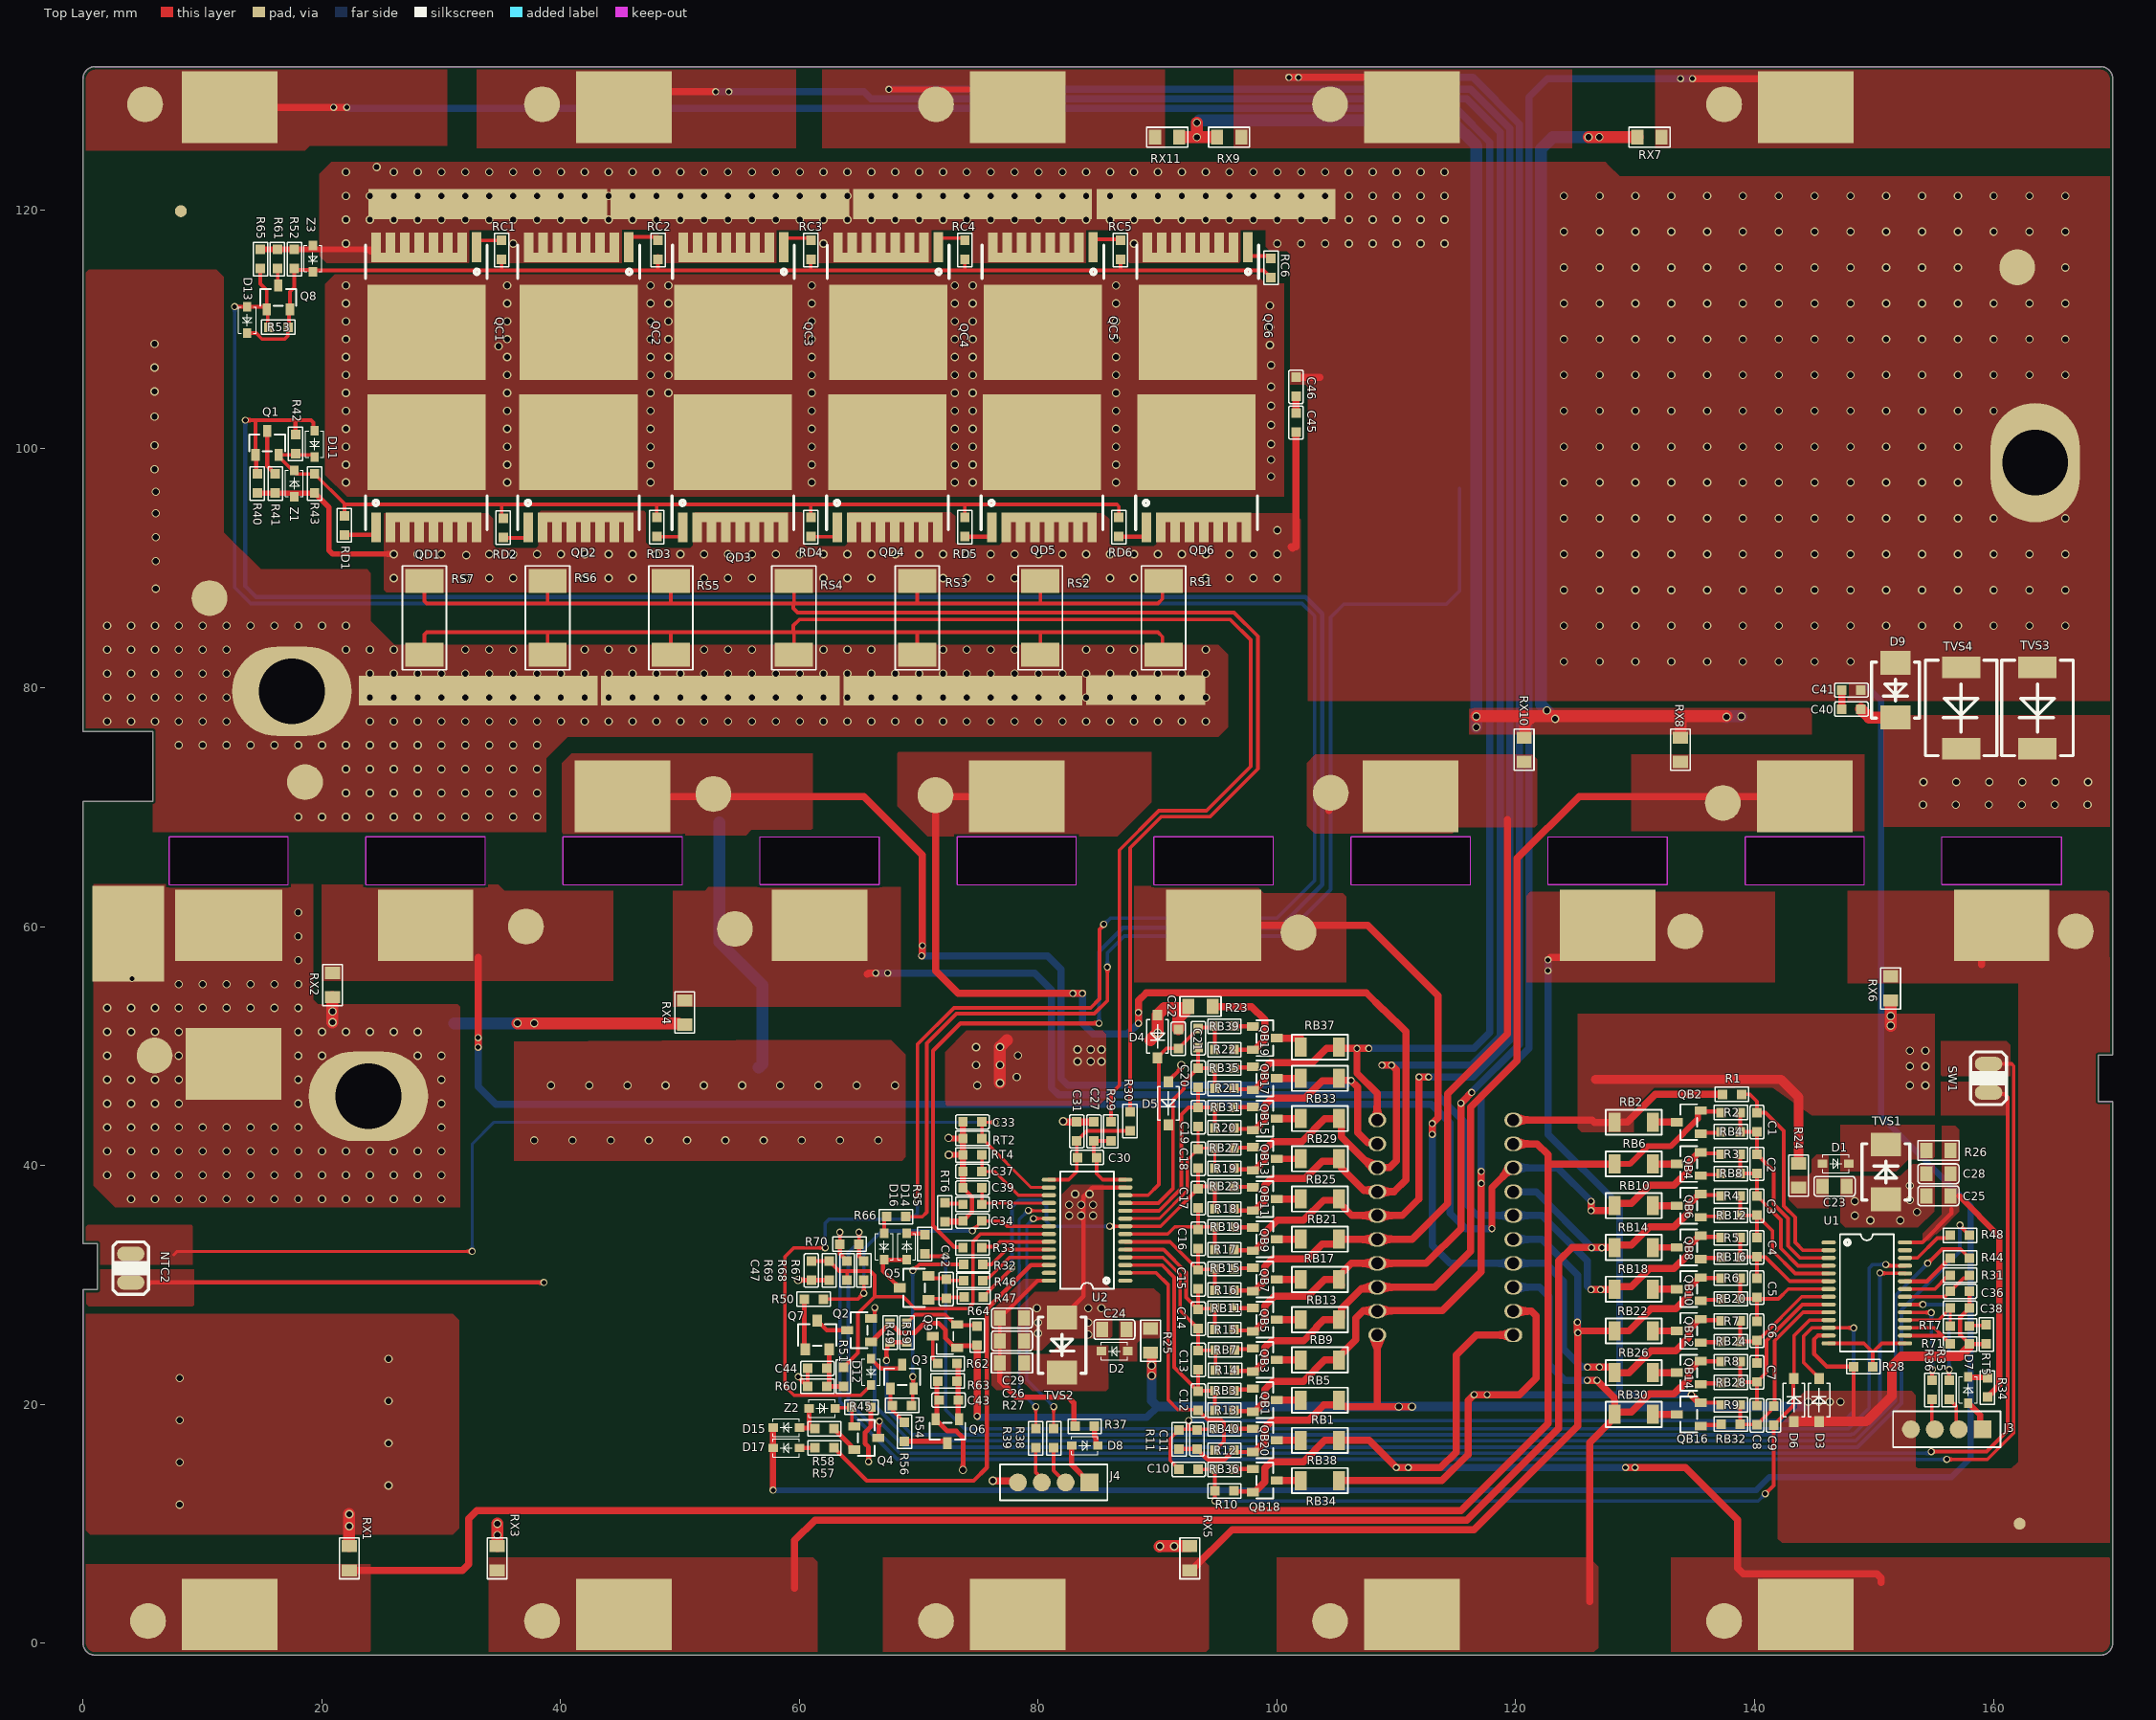
[diagram p0: Top Layer view]
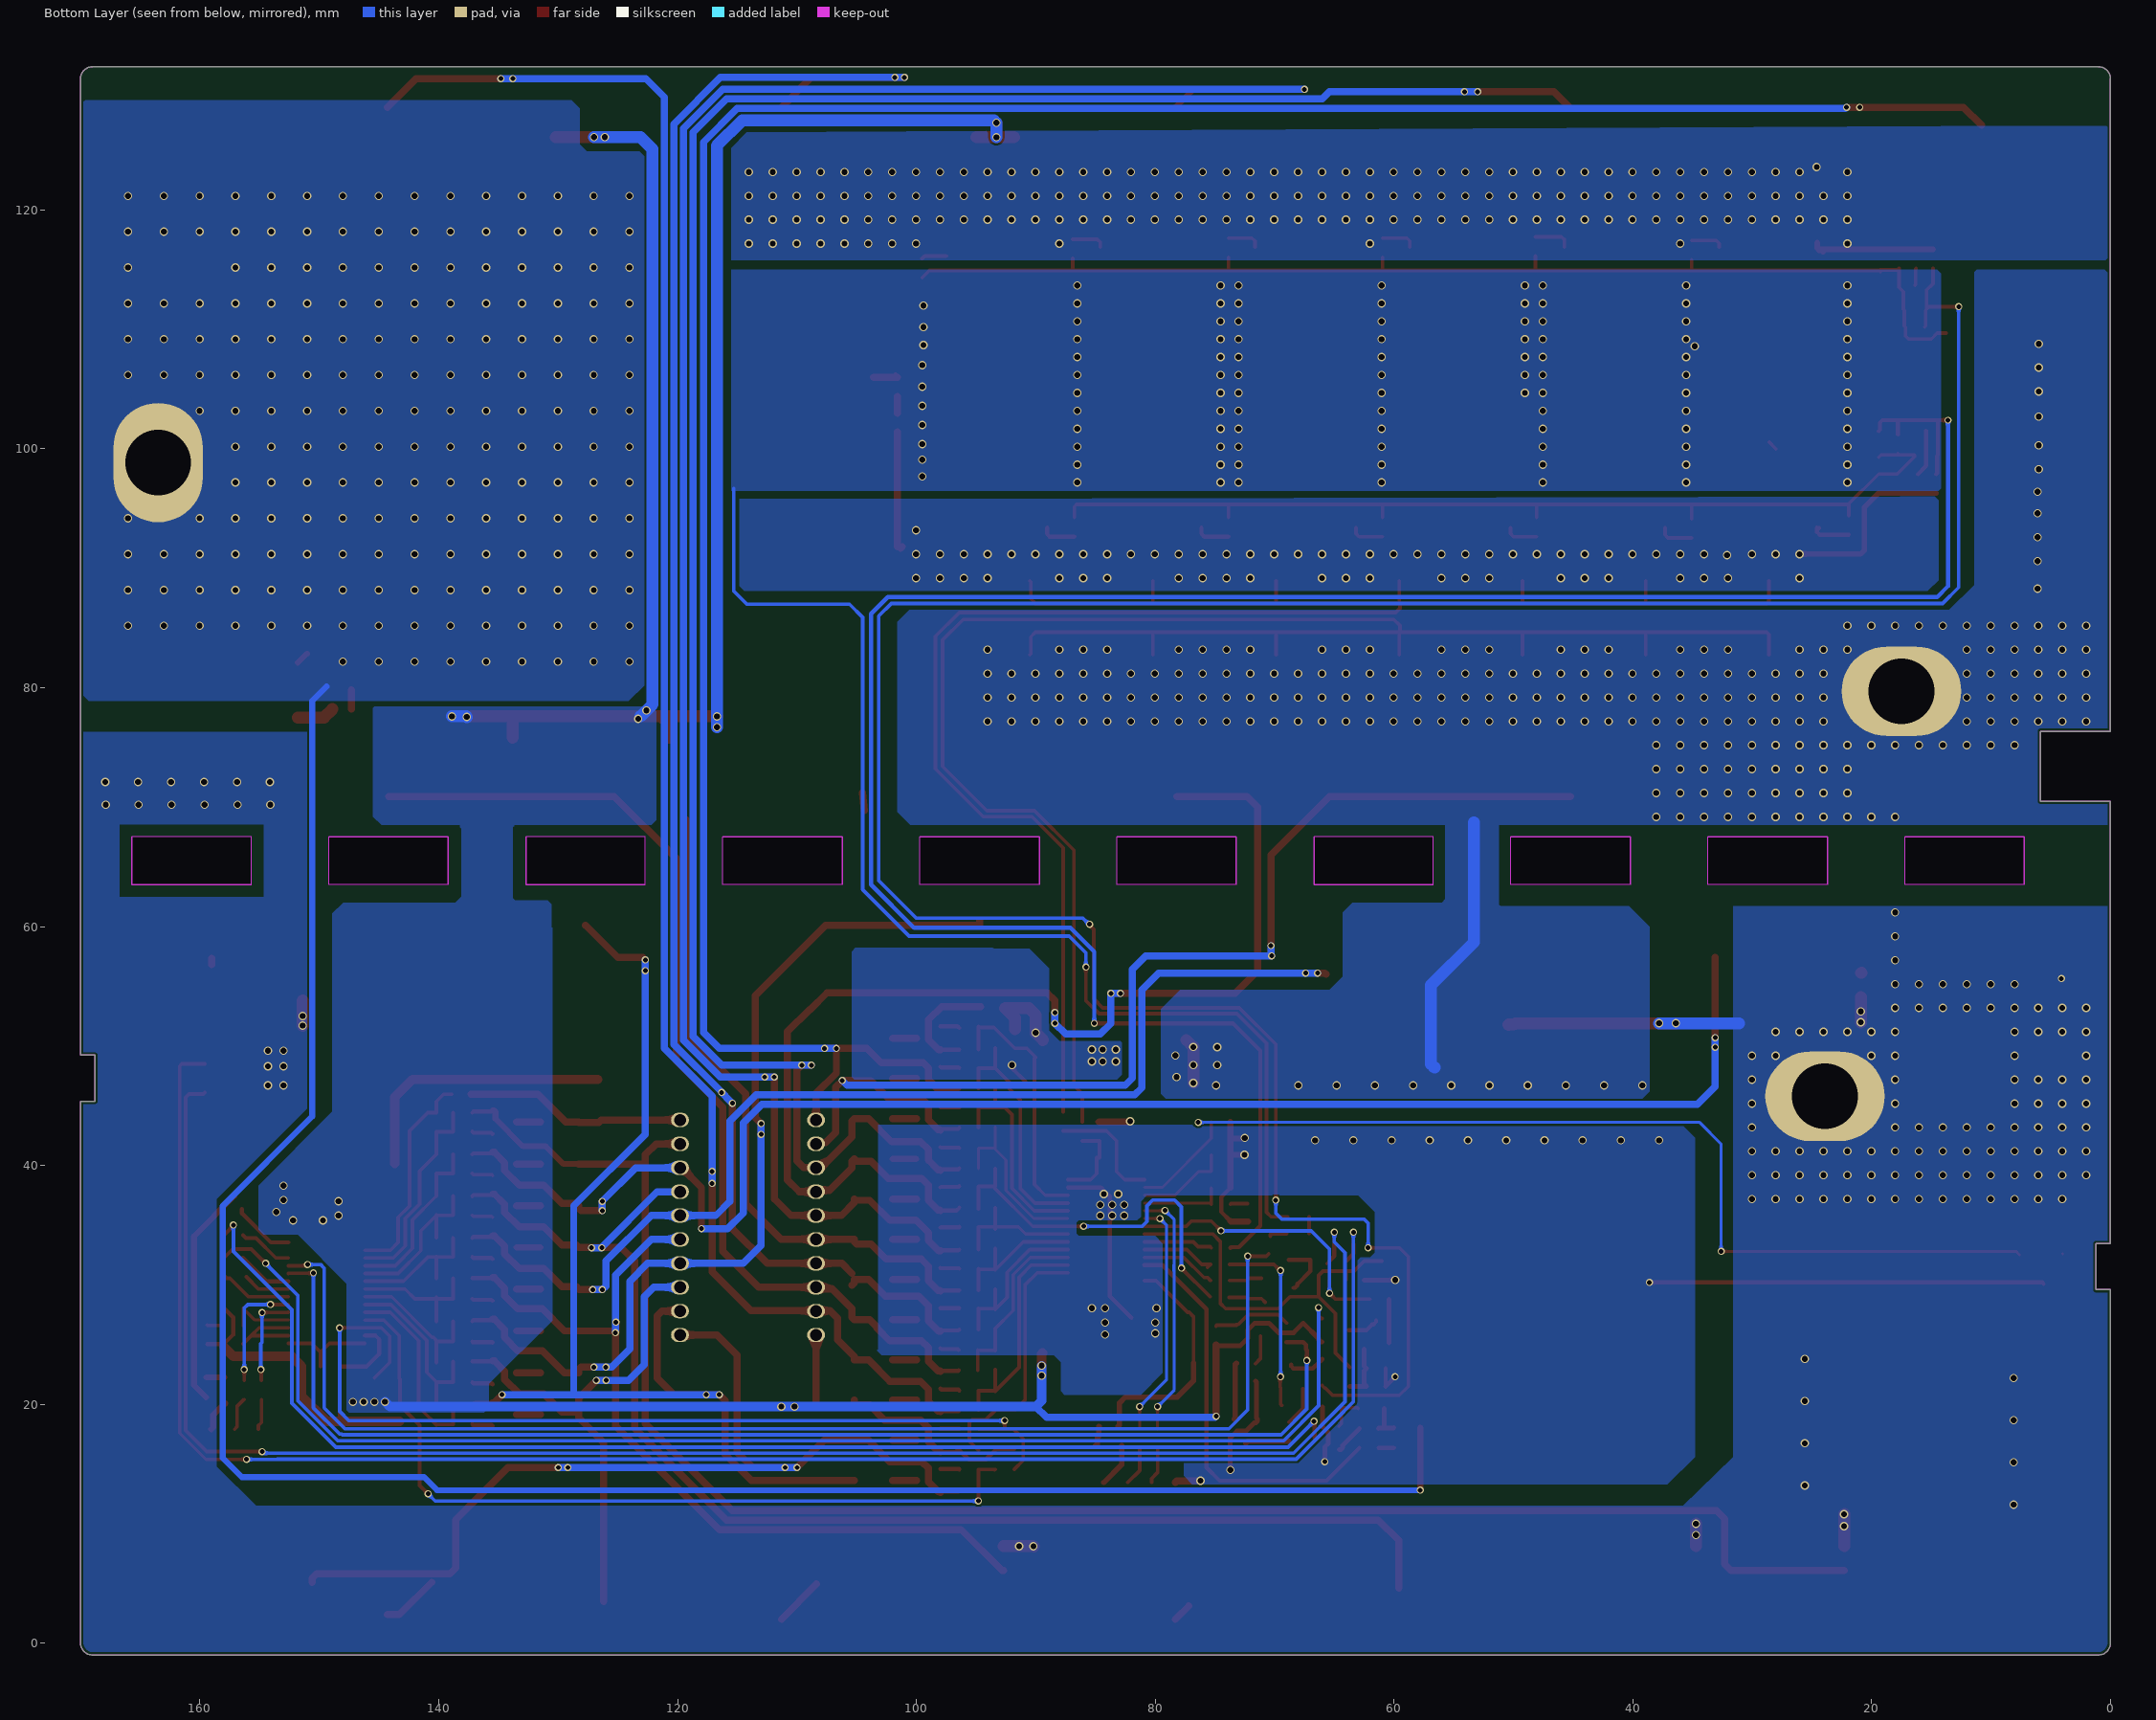
[diagram p1: Bottom Layer view, seen from below]
# Altium PCB MISC82749.PcbDoc (part 1 of 4)
Units mm, origin at the board's own origin, x right, y up, seen from the top; angles counter-clockwise.
Board outline 170 x 133 mm, 2 copper layers (Top Layer, Bottom Layer); 262 components, 170 nets, 783 pads, 1052 vias.

## Layer stack, top to bottom (the 12.6 mil dielectric is the usual default, probably not edited)
Top Solder: solder mask 0.0102, Solder Resist, Dk 3.5
Top Layer: signal copper 0.0356
Dielectric 1: dielectric 0.32, FR-4, Dk 4.8
Bottom Layer: signal copper 0.0356
Bottom Solder: solder mask 0.0102, Solder Resist, Dk 3.5

## Board outline
0,0 0,29.6 1.2,29.6 1.2,33.45 0,33.45 0,70.5 5.85,70.5 5.85,76.35 0,76.35 0,131 cw(c1,131) 1,132 169,132 cw(c169,131) 170,131 170,49.225 168.8,49.225 168.8,45.375 170,45.375 170,0 cw(c169,0) 169,-1 1,-1 cw(c1,0)
cut-out: 155.7,63.5 155.7,67.5 165.7,67.5 165.7,63.5
cut-out: 149.2,63.5 149.2,67.5 139.2,67.5 139.2,63.5
cut-out: 122.7,63.5 122.7,67.5 132.7,67.5 132.7,63.5
cut-out: 106.2,63.5 116.2,63.5 116.2,67.5 106.2,67.5
cut-out: 89.7,63.5 99.7,63.5 99.7,67.5 89.7,67.5
cut-out: 56.7,63.5 56.7,67.5 66.7,67.5 66.7,63.5
cut-out: 73.2,63.5 83.2,63.5 83.2,67.5 73.2,67.5
cut-out: 40.2,63.5 50.2,63.5 50.2,67.5 40.2,67.5
cut-out: 23.7,63.5 33.7,63.5 33.7,67.5 23.7,67.5
cut-out: 7.2,63.5 17.2,63.5 17.2,67.5 7.2,67.5

## Design rules (kind name [scope] priority, off if disabled: settings)
Clearance [All] p1: gap=0.2 ignorepadtopadclearanceinfootprint=FALSE
ComponentClearance [All] p1: gap=0.2 collisioncheckmode=3 verticalgap=0.2 showdistances=FALSE
HoleSize [All] p1: absolutevalues=TRUE maxlimit=50 minlimit=0.025 maxpercent=80.000 minpercent=20.000
PolygonConnect [All] p1: connectstyle=Direct reliefconductorwidth=0.254 reliefentries=4 polygonreliefangle="90 Angle" airgapwidth=0.254
RoutingVias [All] p1: holewidth=0.4 width=0.6 viastyle="Through Hole" minholewidth=0.4 minwidth=0.6 maxholewidth=0.5 maxwidth=7
SolderMaskExpansion [All] p1: expansion=0.102 istentingtop=FALSE
SupplyNets "Schematic Supply Nets_3" [InNet('B0')] p1: voltage=0.000
SupplyNets "Schematic Supply Nets_2" [InNet('P-/C-')] p2: voltage=0.000
SupplyNets "Schematic Supply Nets_1" [InNet('GND')] p3: voltage=0.000
SupplyNets "Schematic Supply Nets" [InNet('B10')] p4: voltage=0.000
Width [All] p1: maxlimit=2 minlimit=0.2 preferedwidth=0.25
28 further rules are at their usual default settings.

## Components (designator, comment, footprint, x,y, rotation, side; value= is the part's Value field where it differs from the comment)
C1 "0.1uF50V" C0603A 140.2,43.618 r90 top
C2 "0.1uF50V" C0603A 140.2,40.127 r90 top
C3 "0.1uF50V" C0603A 140.2,36.636 r90 top
C4 "0.1uF50V" C0603A 140.2,33.145 r90 top
C5 "0.1uF50V" C0603A 140.2,29.755 r90 top
C6 "0.1uF50V" C0603A 140.2,26.15 r90 top
C7 "0.1uF50V" C0603A 140.2,22.673 r90 top
C8 "0.1uF50V" C0603A 140.2,19.082 r90 top
C9 "0.1uF50V" C0603A 141.6,19.05 r90 top
C10 "0.1uF50V" C0603A 92.6,14.55 r0 top
C11 "1uF50V" C0603A 93.3,17.05 r90 top
C12 "0.1uF50V" C0603A 93.4,20.3 r270 top
C13 "0.1uF50V" C0603A 93.4,23.7 r270 top
C14 "0.1uF50V" C0603A 93.4,27.15 r270 top
C15 "0.1uF50V" C0603A 93.4,30.45 r270 top
C16 "0.1uF50V" C0603A 93.4,33.85 r270 top
C17 "0.1uF50V" C0603A 93.4,37.25 r270 top
C18 "0.1uF50V" C0603A 93.4,40.55 r270 top
C19 "0.1uF50V" C0603A 93.4,44.05 r270 top
C20 "0.1uF50V" C0603A 93.4,47.35 r270 top
C21 "0.1uF50V" C0603A 93.4,50.65 r270 top
C22 "1uF50V" C0603A 91.75,50.6 r270 top
C23 "1uF100V" C0805L 146.7,38.25 r180 top
C24 "1uF100V" C0805L 86.384,26.25 r0 top
C25 "1uF100V" C0805L 155.4,37.45 r0 top
C26 "1uF100V" C0805L 77.81,25.31 r180 top
C27 "1uF25V" C0603A 84.667,42.85 r90 top
C28 "0.1uF100V" C0805L 155.4,39.3 r0 top
C29 "0.1uF100V" C0805L 77.81,27.21 r180 top
C30 "1nF25V" C0603A 84.1,40.65 r0 top
C31 "1uF25V" C0603A 83.233,42.85 r270 top
C33 "1nF25V" C0603A 74.5,43.64 r180 top
C34 "1uF25V" C0603A 74.5,35.34 r0 top
C36 "1uF25V" C0603A 157.2,29.45 r180 top
C37 "1nF25V" C0603A 74.5,39.5 r180 top
C38 "1nF25V" C0603A 157.2,28.05 r0 top
C39 "1nF25V" C0603A 74.5,38.12 r180 top
C40 "0.1uF50V" C0603A 148.1,78.2 r0 top
C41 "0.1uF50V" C0603A 148.1,79.8 r180 top
C42 "10nF25V" C0603A 72.3,29.65 r90 top
C43 "0.1uF50V" C0603A 72.5,20.35 r0 top
C44 "1nF25V" C0603A 61.5,23 r180 top
C45 "0.1uF100V" C0603A 101.6,102.2 r270 top
C46 "0.1uF100V" C0603A 101.6,105.2 r270 top
C47 "1nF25V" C0603A 61,31.2 r90 top
D1 "BAV21W" SOD323A 146.8,40.15 r180 top
D2 "BAV21W" SOD323A 86.4,24.45 r0 top
D3 "BAT46W" SOD123 145.4,20.35 r270 top
D4 "BAT46W" SOD123 90,50.8 r90 top
D5 "BAT46W" SOD123 90.9,45.2 r90 top
D6 "BAT46W" SOD123 143.3,20.35 r270 top
D7 "BAV21W" SOD323A 157.9,21.2 r270 top
D8 "BAV21W" SOD323A 83.9,16.55 r180 top
D9 "RS3M" "SMB A" 151.8,79.8 r90 top
D11 "BAV21W" SOD323A 19.4,100.4 r90 top
D12 "BAV21W" SOD323A 66,22.7 r90 top
D13 "BAV21W" SOD323A 13.76,110.792 r90 top
D14 "BAV21W" SOD323A 69,33.2 r270 top
D15 "BAV21W" SOD323A 58.9,18.05 r0 top
D16 "BAV21W" SOD323A 67.1,33.2 r90 top
D17 "BAV21W" SOD323A 58.9,16.35 r0 top
J3 "CH-2.0-4P" Test2.0-4P 156.1,17.9 r180 top
J4 "CH-2.0-4P" Test2.0-4P 81.3,13.45 r180 top
NTC2 "10K B=3435" RT2.3X1.2-2 4,31.4 r270 top
Q1 "MMBT5401" SOT23-3 15.425,100.5 r0 top
Q2 "MMBT5401" SOT23-3 65,26.2 r90 top
Q3 "MMBT5401" SOT23-3 68.6,22.3 r0 top
Q4 "MMBT5551" SOT23-3 65.6,17.175 r270 top
Q5 "AM2394" SOT23-3L 69.6,29.75 r90 top
Q6 "MMBT5551" SOT23-3 72.4,17.75 r180 top
Q7 "AM2394" SOT23-3L 61.5,25.8 r0 top
Q8 "MMBT5401" SOT23-3 16.36,112.676 r0 top
Q9 "MMBT5401" SOT23-3 72.2,25.7 r90 top
QB1 "MMBT5551" SOT23-3 98.984,20.345 r270 top
QB2 "MMBT5551" SOT23-3 134.5,43.618 r90 top
QB3 "MMBT5551" SOT23-3 98.984,23.714 r270 top
QB4 "MMBT5551" SOT23-3 134.5,40.122 r90 top
QB5 "MMBT5551" SOT23-3 98.984,27.082 r270 top
QB6 "MMBT5551" SOT23-3 134.5,36.627 r90 top
QB7 "MMBT5551" SOT23-3 98.984,30.45 r270 top
QB8 "MMBT5551" SOT23-3 134.5,33.131 r90 top
QB9 "MMBT5551" SOT23-3 98.984,33.818 r270 top
QB10 "MMBT5551" SOT23-3 134.5,29.636 r90 top
QB11 "MMBT5551" SOT23-3 98.984,37.186 r270 top
QB12 "MMBT5551" SOT23-3 134.5,26.141 r90 top
QB13 "MMBT5551" SOT23-3 98.984,40.555 r270 top
QB14 "MMBT5551" SOT23-3 134.5,22.645 r90 top
QB15 "MMBT5551" SOT23-3 98.984,43.923 r270 top
QB16 "MMBT5551" SOT23-3 134.5,19.15 r90 top
QB17 "MMBT5551" SOT23-3 98.984,47.291 r270 top
QB18 "MMBT5551" SOT23-3 98.984,13.609 r270 top
QB19 "MMBT5551" SOT23-3 98.984,50.659 r270 top
QB20 "MMBT5551" SOT23-3 98.984,16.977 r270 top
QC1 "N MOS*" TOLL_123 28.76,113.25 r180 top
QC2 "N MOS*" TOLL_123 41.52,113.25 r180 top
QC3 "N MOS*" TOLL_123 54.48,113.25 r180 top
QC4 "N MOS*" TOLL_123 67.44,113.25 r180 top
QC5 "N MOS*" TOLL_123 80.4,113.25 r180 top
QC6 "N MOS*" TOLL_123 93.36,113.25 r180 top
QD1 "N MOS*" TOLL_123 28.76,97.05 r0 top
QD2 "N MOS*" TOLL_123 41.5,97.05 r0 top
QD3 "N MOS*" TOLL_123 54.44,97.05 r0 top
QD4 "N MOS*" TOLL_123 67.38,97.05 r0 top
QD5 "N MOS*" TOLL_123 80.32,97.05 r0 top
QD6 "N MOS*" TOLL_123 93.26,97.05 r0 top
R1 "510R" R0603A 138.1,45.95 r0 top
R2 "510R" R0603A 138,44.418 r0 top
R3 "510R" R0603A 138,40.927 r0 top
R4 "510R" R0603A 138,37.436 r0 top
R5 "510R" R0603A 138,33.945 r0 top
R6 "510R" R0603A 138,30.555 r0 top
R7 "510R" R0603A 138,26.964 r0 top
R8 "510R" R0603A 138,23.573 r0 top
R9 "510R" R0603A 138,19.95 r0 top
R10 "510R" R0603A 95.6,12.75 r180 top
R11 "510R" R0603A 91.8,17.05 r90 top
R12 "510R" R0603A 95.6,16.15 r180 top
R13 "510R" R0603A 95.6,19.5 r180 top
R14 "510R" R0603A 95.65,22.85 r180 top
R15 "510R" R0603A 95.6,26.25 r180 top
R16 "510R" R0603A 95.6,29.55 r180 top
R17 "510R" R0603A 95.6,32.95 r180 top
R18 "510R" R0603A 95.6,36.35 r180 top
R19 "510R" R0603A 95.6,39.75 r180 top
R20 "510R" R0603A 95.6,43.15 r180 top
R21 "510R" R0603A 95.6,46.45 r180 top
R22 "510R" R0603A 95.6,49.7 r180 top
R23 "510R" R0805L 93.6,53.3 r0 top
R24 "1K" R0805L 143.7,39.15 r90 top
R25 "1K" R0805L 89.41,25.326 r270 top
R26 "100R" R0805L 155.4,41.25 r180 top
R27 "100R" R0805L 77.81,23.46 r0 top
R28 "1K" R0603A 149.1,23.15 r0 top
R29 "10R" R0603A 86.1,42.85 r270 top
R30 "10R" R0603A 87.7,43.7 r90 top
R31 "1K" R0603A 157.2,30.8 r180 top
R32 "1K" R0603A 74.56,31.71 r180 top
R33 "1K" R0603A 74.5,33.1 r180 top
R34 "100R" R0603A 159.5,21.4 r90 top
R35 "100R" R0603A 156.3,21.2 r270 top
R36 "100R" R0603A 154.85,21.2 r270 top
R37 "100R" R0603A 83.9,18.15 r0 top
R38 "100R" R0603A 81.3,17.15 r270 top
R39 "100R" R0603A 79.8,17.15 r270 top
R40 "5.1M" R0603A 14.6,97.1 r270 top
R41 "510R" R0603A 16.1,97.1 r270 top
R42 "0R/NC*" R0603A 17.8,100.4 r270 top
R43 "5.1M" R0603A 19.4,97.1 r270 top
R44 "1M" R0603A 157.2,32.25 r180 top
R45 "510K" R0603A 65.2,19.75 r180 top
R46 "10K" R0603A 74.56,30.36 r0 top
R47 "10K" R0603A 74.6,29 r0 top
R48 "10M" R0603A 157.2,34.15 r180 top
R49 "1M" R0603A 67.6,26 r90 top
R50 "100K" R0603A 61.2,28.8 r0 top
R51 "100K" R0603A 63.7,22.3 r90 top
R52 "5.1M" R0603A 17.7,115.9 r90 top
R53 "0R/NC*" R0603A 16.36,110.192 r0 top
R54 "1M" R0603A 68.6,19.9 r0 top
R55 "1M" R0603A 70.5,33.4 r270 top
R56 "3M" R0603A 68.8,17.7 r270 top
R57 "3M" R0603A 62.1,16.35 r0 top
R58 "1M" R0603A 62.1,17.95 r0 top
R59 "3M" R0603A 69,26 r270 top
R60 "10M" R0603A 61.5,21.5 r0 top
R61 "510R" R0603A 16.28,115.9 r90 top
R62 "3M" R0603A 72.4,23.4 r180 top
R63 "1M" R0603A 72.4,21.95 r180 top
R64 "1M" R0603A 74.9,25.75 r270 top
R65 "5.1M" R0603A 14.86,115.9 r90 top
R66 "1M" R0603A 68.1,35.7 r180 top
R67 "100K" R0603A 65.4,31.2 r270 top
R68 "100K" R0603A 64,31.2 r90 top
R69 "10M" R0603A 62.5,31.2 r270 top
R70 "100K" R0603A 64.2,33.4 r0 top
R71 "10K" R0603A 157.2,25.05 r180 top
RB1 "100R" R1206A 103.6,20.345 r180 top
RB2 "100R" R1206A 129.884,43.618 r0 top
RB3 "510R" R0603A 95.6,21.15 r180 top
RB4 "510R" R0603A 138,42.818 r0 top
RB5 "100R" R1206A 103.6,23.714 r180 top
RB6 "100R" R1206A 129.884,40.122 r0 top
RB7 "510R" R0603A 95.65,24.55 r180 top
RB8 "510R" R0603A 138,39.32 r0 top
RB9 "100R" R1206A 103.6,27.082 r180 top
RB10 "100R" R1206A 129.884,36.627 r0 top
RB11 "510R" R0603A 95.6,28.05 r180 top
RB12 "510R" R0603A 138,35.822 r0 top
RB13 "100R" R1206A 103.6,30.45 r180 top
RB14 "100R" R1206A 129.884,33.131 r0 top
RB15 "510R" R0603A 95.6,31.35 r180 top
RB16 "510R" R0603A 138,32.324 r0 top
RB17 "100R" R1206A 103.6,33.818 r180 top
RB18 "100R" R1206A 129.884,29.636 r0 top
RB19 "510R" R0603A 95.6,34.85 r180 top
RB20 "510R" R0603A 138,28.826 r0 top
RB21 "100R" R1206A 103.6,37.186 r180 top
RB22 "100R" R1206A 129.884,26.141 r0 top
RB23 "510R" R0603A 95.6,38.25 r180 top
RB24 "510R" R0603A 138,25.25 r0 top
RB25 "100R" R1206A 103.6,40.555 r180 top
RB26 "100R" R1206A 129.884,22.645 r0 top
RB27 "510R" R0603A 95.6,41.45 r180 top
RB28 "510R" R0603A 138,21.83 r0 top
RB29 "100R" R1206A 103.6,43.923 r180 top
RB30 "100R" R1206A 129.884,19.15 r0 top
RB31 "510R" R0603A 95.6,44.85 r180 top
RB32 "510R" R0603A 138,18.332 r0 top
RB33 "100R" R1206A 103.6,47.291 r180 top
RB34 "100R" R1206A 103.6,13.609 r180 top
RB35 "510R" R0603A 95.6,48.15 r180 top
RB36 "510R" R0603A 95.6,14.55 r180 top
RB37 "100R" R1206A 103.6,49.9 r180 top
RB38 "100R" R1206A 103.6,16.977 r180 top
RB39 "510R" R0603A 95.6,51.65 r180 top
RB40 "510R" R0603A 95.6,17.95 r180 top
RC1 "47R" R0603A 35.06,116.65 r90 top
RC2 "47R" R0603A 48.16,116.65 r270 top
RC3 "47R" R0603A 60.96,116.65 r270 top
RC4 "47R" R0603A 73.86,116.65 r90 top
RC5 "47R" R0603A 86.9,116.65 r90 top
RC6 "47R" R0603A 99.5,115.15 r90 top
RD1 "47R" R0603A 21.9,93.6 r270 top
RD2 "47R" R0603A 35.2,93.4 r270 top
RD3 "47R" R0603A 48.06,93.45 r270 top
RD4 "47R" R0603A 60.96,93.45 r90 top
RD5 "47R" R0603A 73.86,93.45 r90 top
RD6 "47R" R0603A 86.76,93.45 r90 top
RS1 "R010" R2512L 90.5,85.85 r90 top
RS2 "R010" R2512L 80.183,85.85 r90 top
RS3 "R010" R2512L 69.867,85.85 r90 top
RS4 "R010" R2512L 59.55,85.85 r90 top
RS5 "R010" R2512L 49.233,85.85 r90 top
RS6 "R010" R2512L 38.917,85.85 r90 top
RS7 "R010" R2512L 28.6,85.85 r90 top
RT2 "10K B=3435" R0603A 74.5,42.26 r180 top
RT4 "10K B=3435" R0603A 74.5,40.88 r180 top
RT5 "10K B=3435" R0603A 159.4,25.85 r270 top
RT6 "10K B=3435" R0603A 72.19,36.07 r270 top
RT7 "0R" R0603A 157.2,26.55 r180 top
RT8 "0R" R0603A 74.5,36.74 r0 top
RX1 "0R" R0805L 22.3,7.1 r270 top
RX2 "0R" R0805L 20.9,55.1 r90 top
RX3 "0R" R0805L 34.7,7.1 r270 top
RX4 "0R" R0805L 50.4,52.8 r90 top
RX5 "0R" R0805L 92.7,7.1 r270 top
RX6 "0R" R0805L 151.4,54.816 r270 top
RX7 "0R" R0805L 131.2,126.1 r0 top
RX8 "0R" R0805L 133.8,74.8 r270 top
RX9 "0R" R0805L 96,126.1 r0 top
RX10 "0R" R0805L 120.7,74.8 r270 top
RX11 "0R" R0805L 90.8,126.1 r180 top
SW1 "SW_1" RT2.3X1.2-2 159.6,47.3 r90 top
TVS1 "SMBJ64A" "SMB A" 151,39.45 r270 top
TVS2 "SMBJ64A" "SMB A" 82,24.95 r90 top
TVS3 "SMBJ75A*" SMC_MDO-214AB) 163.7,78.3 r270 top
TVS4 "SMBJ75A*" SMC_MDO-214AB) 157.3,78.3 r270 top
U1 "SH3676010" TSSOP-28L(PIN间距0.65mm) 149.4,29.325 r0 top
U2 "SH3676010" TSSOP-28L(PIN间距0.65mm) 84.1,34.575 r180 top
Z1 "15V" SOD323A 17.7,97.1 r270 top
Z2 "3.3V" SOD323A 61.9,19.65 r180 top
Z3 "15V" SOD323A 19.26,115.942 r90 top

## Footprints (in the part's own frame and the unit in brackets; to place one, negate y for a bottom-side part, rotate by r counter-clockwise, add the part's x,y. Pads: shape width x height; smd on the part's side, far side on the other; paste and mask are expansions set on the pad)
C0603A [mm] "贴片电容"
  rect 0.8x0.8 smd mask+0.08: 1(-0.8,0) 2(0.8,0)
  silkscreen extent -1.4,-0.6 1.4,0.6
C0805L [mil] "贴片电容"
  rect 40x50 smd paste+0 mask+1.97: 1(-40,0) 2(40,0)
  silkscreen extent -68,-32 68,32
R0603A [mm] "贴片电阻"
  rect 0.8x0.8 smd mask+0.08: 1(-0.8,0) 2(0.8,0)
  silkscreen extent -1.4,-0.6 1.4,0.6
R0805L [mil] "贴片电阻"
  rect 40x50 smd paste+0 mask+1.97: 1(-40,0) 2(40,0)
  silkscreen extent -68,-32 68,32
R1206A [mm] "贴片电阻"
  rect 1x1.6 smd: 1(-1.6,0) 2(1.6,0)
  silkscreen extent -2.35,-1.05 2.35,1.05
R2512L [mm] "贴片电阻"
  rect 2x3.2 smd: 1(-3.1,0) 2(3.1,0)
  silkscreen extent -4.35,-1.85 4.35,1.85
RT2.3X1.2-2 [mm] "焊线NTC"
  oval 1.2x2.3 smd: 1(-1.2,0) 2(1.2,0)
  silkscreen extent -2.2,-1.55 2.2,1.5
"SMB A" [mm] "贴片二极管"
  rect 2x2.5 smd: 1(-2.3,0) 2(2.3,0)
  silkscreen extent -2.35,-2 2.35,2
SMC_MDO-214AB) [mm] "贴片二极管"
  rect 1.8x3.2 smd: 1(-3.4,0) 2(3.4,0)
  silkscreen extent -4,-3 4,3
SOD123 [mm] "贴片二极管"
  rect 0.9x0.8 smd: 1(-1.8,0) 2(1.8,0)
  silkscreen extent -1.4,-0.9 1.4,0.9
SOD323A [mm] "贴片二极管"
  rect 0.8x0.7 smd: 1(-1.1,0) 2(1.1,0)
  silkscreen extent -1.1,-0.75 1.1,0.75
SOT23-3 [mm] "贴片IC/MOS*"
  rect 0.7x1 smd: 1(-0.975,-1) 2(0.975,-1) 3(0,1.016)
  silkscreen extent -1.5,-0.7 1.5,0.7
SOT23-3L [mm] "贴片IMOS"
  rect 0.8x1 smd: 1(-1,-1.2) 2(1,-1.2) 3(0,1.2)
  silkscreen extent -1.6,-0.9 1.6,0.9
Test2.0-4P [mm] "测试座2.0mm"
  rect 1.5x1.5 smd: 1(-3,0)
  round 1.5 smd: 2(-1,0) 3(1,0) 4(3,0)
  silkscreen extent -4.5,-1.5 4.5,1.5
TOLL_123 [mm] "贴片MOS"
  rect 0.8x2.5 smd: 1(-4.2,-3.638)
  rect 0.8x1.7 smd: 2(-3,-4) 2(-1.8,-4) 2(-0.6,-4) 2(0.6,-4) 2(1.8,-4) 2(3,-4) 2(4.2,-4)
  rect 8x0.8 smd: 2(0.6,-2.788)
  rect 9.9x8 smd: 3(0,3.5)
  silkscreen extent -5.1,-3.8 5.1,-1
TSSOP-28L(PIN间距0.65mm) [mm] "贴片IC"
  oval 1.2x0.35 smd: 1(-3.2,4.225) 2(-3.2,3.575) 3(-3.2,2.925) 4(-3.2,2.275) 5(-3.2,1.625) 6(-3.2,0.975) 7(-3.2,0.325) 8(-3.2,-0.325) 9(-3.2,-0.975) 10(-3.2,-1.625) 11(-3.2,-2.275) 12(-3.2,-2.925) 13(-3.2,-3.575) 14(-3.2,-4.225) 15(3.2,-4.225) 16(3.2,-3.575) 17(3.2,-2.925) 18(3.2,-2.275) 19(3.2,-1.625) 20(3.2,-0.975) 21(3.2,-0.325) 22(3.2,0.325) 23(3.2,0.975) 24(3.2,1.625) 25(3.2,2.275) 26(3.2,2.925) 27(3.2,3.575) 28(3.2,4.225)
  silkscreen extent -2.25,-4.9 2.25,4.9

## Part data
C1 C2 C3 C4 C5 C6 C7 C8 C9 C10 C11 C12 C13 C14 C15 C16 C17 C18 C19 C20 C21 C22 C23 C24 C25 C26 C27 C28 C29 C30 C31 C33 C34 C36 C37 C38 C39 C40 C41 C42 C43 C44 C45 C46 C47: library part CAP, "SMD capacitor"
D1 D2 D7 D8 D11 D12 D13 D14 D15 D16 D17: library part BAV21_SOD323, "SMD diode"
D3 D4 D5 D6: library part BAT46W_SOD123, "SMD diode"
D9: "SMD diode"
J3 J4: library part Test2.0-4P, "test socket"
NTC2 RT2 RT4 RT5 RT6: library part NTC, "SMD thermistor"
Q1 Q2 Q3 Q4 Q6 Q8 Q9 QB1 QB2 QB3 QB4 QB5 QB6 QB7 QB8 QB9 QB10 QB11 QB12 QB13 QB14 QB15 QB16 QB17 QB18 QB19 QB20: "SMD transistor"
Q5 Q7: library part AM2394_VGS100V, "SMD N MOS_VGS100V"
QC1 QC2 QC3 QC4 QC5 QC6 QD1 QD2 QD3 QD4 QD5 QD6: "SMD MOSFET"
R1 R2 R3 R4 R5 R6 R7 R8 R9 R10 R11 R12 R13 R14 R15 R16 R17 R18 R19 R20 R21 R22 R28 R29 R30 R31 R32 R33 R34 R35 R36 R37 R38 R39 R40 R41 R42 R43 R44 R45 R46 R47 R48 R49 R50 R51 R52 R53 R54 R55 R56 R57 R58 R59 R60 R61 R62 R63 R64 R65 R66 R67 R68 R69 R70 R71 RB3 RB4 RB7 RB8 RB11 RB12 RB15 RB16 RB19 RB20 RB23 RB24 RB27 RB28 RB31 RB32 RB35 RB36 RB39 RB40 RC1 RC2 RC3 RC4 RC5 RC6 RD1 RD2 RD3 RD4 RD5 RD6 RT7 RT8: library part RES, "SMD resistor"
R23 R24 R25 R26 R27 RX1 RX2 RX3 RX4 RX5 RX6 RX7 RX8 RX9 RX10 RX11: library part RES_0805, "SMD resistor"
RB1 RB2 RB5 RB6 RB9 RB10 RB13 RB14 RB17 RB18 RB21 RB22 RB25 RB26 RB29 RB30 RB33 RB34 RB37 RB38: library part RES3, "alloy SMD resistor"
RS1 RS2 RS3 RS4 RS5 RS6 RS7: library part RES2_2512, "SMD alloy resistor"
SW1: "soft-touch switch"
TVS1 TVS2: "SMD diode (ESD and surge protection)"
TVS3 TVS4: library part "TVS C", "SMD diode (ESD and surge protection)"
Z1 Z3: library part "15V SOD323", "SMD zener diode"
Z2: library part 3.3_SOD323, "SMD zener diode"

## Free pads (board coordinates)
  oval 10x7.5 hole 5.5: 66(17.5,79.7) 66(23.904,45.783)
  oval 7.5x10 hole 5.5: 66(163.5,98.85)
  round 1 smd: 74(8.2,119.9) 75(162.2,10)
  rect 6x8 smd: 81(3.8,59.4)
  rect 9x6 smd: 81(12.2,60.1)
  rect 8x6 smd: 81(12.3,2.4) 81(12.3,128.6) 81(12.6,48.5) 81(28.7,60.1) 81(45.2,70.9) 81(45.3,2.4) 81(45.3,128.6) 81(61.7,60.1) 81(78.2,70.9) 81(78.3,2.4) 81(78.3,128.6) 81(94.7,60.1) 81(111.2,70.9) 81(111.3,2.4) 81(111.3,128.6) 81(127.7,60.1) 81(144.2,70.9) 81(144.3,2.4) 81(144.3,128.6) 81(160.7,60.1)
  rect 20x2.5 smd: 82(33.1,79.75) 82(33.9,120.5) 83(53.4,79.75) 83(54.2,120.5) 83(73.7,79.75) 84(74.5,120.5) 85(94.9,120.5)
  rect 10x2.5 smd: 83(89,79.8)
  round 3 smd: 86(5.2,128.85) 86(5.45,1.85) 86(6,49.2) 86(10.6,87.5) 86(18.6,72.1) 86(37.1,60) 86(38.45,1.85) 86(38.45,128.85) 86(52.8,71.1) 86(54.6,59.8) 86(71.4,71) 86(71.45,1.85) 86(71.45,128.85) 86(101.8,59.5) 86(104.45,1.85) 86(104.45,128.85) 86(104.5,71.2) 86(134.2,59.6) 86(137.35,70.35) 86(137.45,1.85) 86(137.45,128.85) 86(162,115.2) 86(166.9,59.6)
  oval 1.5x1.2 hole 1: 89(108.4,27.8) 89(108.4,31.8) 89(108.4,37.8) 89(108.4,39.8) 89(108.4,43.8) 89(119.8,27.8) 89(119.8,31.8) 89(119.8,37.8) 89(119.8,39.8) 90(108.4,25.8) 90(108.4,29.8) 90(108.4,33.8) 90(108.4,35.8) 90(108.4,41.8) 90(119.8,25.8) 90(119.8,29.8) 90(119.8,33.8) 90(119.8,35.8) 90(119.8,41.8) ""(119.8,43.8)

## Via types
v1: diameter 0.7, hole 0.5, Top Layer to Bottom Layer, tented both sides, 953 vias
v2: diameter 0.6, hole 0.4, Top Layer to Bottom Layer, tented both sides, 99 vias

## Nets (pads, with @x,y where several pads share a name; then routed paths per layer and width w, separated by ;. In a path a pad name is that pad's centre, name@x,y a point inside that pad or via, vN(x,y) a via of type N, cw(c..) or ccw(c..) an arc to the next point about the centre after c; other vN are vias at no path point)
B0: QB19.2 R22.1 R23.2 | length 9.4
  Top Layer w0.35: R22.1@96.4,49.7 96.408,49.692 97.976,49.692 QB19.2@97.984,49.684
  Top Layer w0.6: R23.2@94.616,53.3 97.875,53.3 98.984,52.191 98.984,50.534 98.134,49.684 QB19.2@97.984,49.684
B1: pad.81@12.3,128.6 pad.86@5.2,128.85 pad.89@108.4,43.8 QB17.2 R21.1 RB37.1 | length 215.1
  Top Layer w0.35: R21.1@96.4,46.45 96.467,46.383 97.917,46.383 QB17.2@97.984,46.316
  Top Layer w0.6: pad.81@10.8,127.1 pad.81@12.3,128.6 v2(22.1,128.6) ; QB17.2@97.984,46.316 98.034,46.366 98.184,46.366 99,47.182 99,48.149 99.442,48.591 102.945,48.591 104.151,49.797 105.2,49.797 105.203,49.8 v2(106.7,49.8) ; v2(107.7,49.8) v2(106.7,49.8) ; pad.89@108.4,43.8 108.4,46.031 106.7,47.731 v2(106.7,49.8)
  Bottom Layer w0.6: v2(22.1,128.6) 22.2,128.5 115,128.5 117.819,125.681 117.819,51.119 116.5,49.8 v2(107.7,49.8) v2(106.7,49.8)
  other v2: 21,128.6
B2: pad.81@45.2,70.9 pad.86@52.8,71.1 pad.90@108.4,41.8 QB15.2 R20.1 RB33.1 | length 101.2
  Top Layer w0.35: R20.1@96.4,43.15 96.501,43.049 97.883,43.049 QB15.2@97.984,42.948
  Top Layer w0.6: pad.81@45.2,70.9 65.4,70.9 70.3,66 70.3,57.6 v2(70.25,57.55) ; QB15.2@97.984,42.948 98.034,42.998 98.184,42.998 99,43.814 99,45.05 99.585,45.635 102.352,45.635 103.8,47.084 105.2,47.084 105.2,46.991 105.309,47.1 v2(106.2,47.1) 106.75,46.55 106.75,42.75 107.585,41.915 107.973,41.915 108,41.888 pad.90@108,41.8
  Bottom Layer w0.6: v2(70.3,58.4) 70.3,57.6 v2(70.25,57.55) 80.781,57.55 81.9,56.431 81.9,47.3 82.5,46.7 105.8,46.7 v2(106.2,47.1)
B3: pad.81@45.3,128.6 pad.86@38.45,128.85 pad.89@108.4,39.8 QB13.2 R19.1 RB29.1 | length 189.6
  Top Layer w0.35: R19.1@96.4,39.75 96.485,39.665 97.899,39.665 QB13.2@97.984,39.58
  Top Layer w0.6: pad.81@45.3,128.6 46.6,129.9 v2(53,129.9) ; QB13.2@97.984,39.58 98.034,39.63 98.184,39.63 99,40.446 99,41.35 99.656,42.006 102.09,42.006 104.007,43.923 RB29.1@105.2,43.923 105.4,43.723 105.4,42.4 107.885,39.915 108.285,39.915 pad.89@108.4,39.8 108.436,39.836 109.436,39.836 110,40.4 110,48 v2(109.6,48.4) v2(108.8,48.4)
  Bottom Layer w0.6: v2(53,129.9) v2(54.1,129.9) 65.4,129.9 66,129.3 115.9,129.3 118.7,126.5 118.7,50.8 116.3,48.4 v2(108.8,48.4)
B4: pad.81@78.2,70.9 pad.86@71.4,71 pad.89@108.4,37.8 QB11.2 R18.1 RB25.1 | length 100.5
  Top Layer w0.35: R18.1@96.4,36.45 96.639,36.211 QB11.2@97.984,36.211
  Top Layer w0.6: pad.81@78.2,70.9 72.3,70.9 71.4,70 71.4,56.3 73.3,54.4 v2(82.9,54.4) v2(83.7,54.4) ; v2(88.4,51.9) v2(88.4,52.8) 88.4,53.8 89.035,54.435 107.5,54.435 108.9,53.035 ; QB11.2@97.984,36.211 98.034,36.261 98.184,36.261 99,37.077 99,38.35 99.549,38.899 102.352,38.899 103.8,40.347 105,40.347 105.2,40.547 RB25.1@105.2,40.555 105.4,40.355 105.4,39.8 107.285,37.915 107.973,37.915 108,37.888 pad.89@108,37.8 ; pad.89@108.4,37.8 109.8,37.8 110.8,38.8 110.8,51.2 108.932,53.068
  Bottom Layer w0.6: v2(82.9,54.4) v2(83.7,54.4) 83.7,51.9 84.6,51 87.5,51 v2(88.4,51.9) v2(88.4,52.8)
B5: pad.81@78.3,128.6 pad.86@71.45,128.85 pad.90@108.4,35.8 QB9.2 R17.1 RB21.1 RX11.2 | length 180.1
  Top Layer w0.35: R17.1@96.4,32.95 96.453,32.897 97.931,32.897 QB9.2@97.984,32.843
  Top Layer w0.5: v2(67.5,130.1) 76.8,130.1 pad.81@78.3,128.6
  Top Layer w0.6: QB9.2@97.984,32.843 98.134,32.843 99,33.709 99,34.375 100.029,35.404 102.225,35.404 103.902,37.081 105.095,37.081 RB21.1@105.2,37.186 105.2,36.886 106.286,35.8 110.5,35.8 111.9,37.2 v2(111.9,47.4) v2(112.7,47.4)
  Bottom Layer w0.6: v2(67.5,130.1) 116.231,130.1 119.5,126.831 119.5,50.469 116.431,47.4 v2(111.9,47.4)
B6: pad.81@111.2,70.9 pad.86@104.5,71.2 pad.90@108.4,33.8 QB7.2 R16.1 RB17.1 RX10.2 | length 57.5
  Top Layer w0.35: R16.1@96.4,29.55 96.438,29.513 97.947,29.513 QB7.2@97.984,29.475
  Top Layer w0.6: QB7.2@97.984,29.475 98.034,29.525 98.184,29.525 99,30.341 99,31.55 99.605,32.155 102.555,32.155 103.8,33.4 105,33.4 105.2,33.6 RB17.1@105.2,33.818 ; 104.35,69.701 pad.86@104.5,71.2 ; RB17.1@105.218,33.8 pad.90@108.4,33.8 ; pad.90@108.4,33.818 111.318,33.818 114.3,36.8 114.3,46 119.3,51 119.3,68.976
B7: pad.81@111.3,128.6 pad.86@104.45,128.85 pad.89@108.4,31.8 QB5.2 R15.1 RB13.1 RX9.2 | length 151.6
  Top Layer w0.35: R15.1@96.4,26.25 96.472,26.178 97.912,26.178 QB5.2@97.984,26.107
  Top Layer w0.6: QB5.2@97.984,26.107 98.134,26.107 99,26.973 99,28.25 99.794,29.044 102.602,29.044 104.007,30.45 RB13.1@105.2,30.45 105.2,30.15 RB13.1@105.4,29.95 ; v2(101,131.1) v2(101.8,131.1) 108.8,131.1 pad.81@111.3,128.6 ; RB13.1@105.4,30.95 106.25,31.8 pad.89@108.4,31.8 112.5,31.8 115.4,34.7 v2(115.4,45.2) 115.6,45.4 v2(116.3,46.1)
  Bottom Layer w0.6: v2(101,131.1) v2(101.8,131.1) 116.4,131.1 120.3,127.2 120.3,50.137 116.3,46.137 v2(116.3,46.1) 115.6,45.4 v2(115.4,45.2)
B8: pad.81@144.2,70.9 pad.86@137.35,70.35 pad.90@108.4,29.8 QB3.2 R14.1 RB9.1 RX8.2 | length 85.9
  Top Layer w0.35: R14.1@96.45,22.85 96.506,22.794 97.928,22.794 QB3.2@97.984,22.739
  Top Layer w0.6: QB3.2@97.984,22.739 98.034,22.789 98.184,22.789 99,23.605 99,24.75 99.574,25.324 102.25,25.324 103.319,26.394 103.319,26.469 103.932,27.082 RB9.1@105.2,27.082 105.4,27.282 105.4,28 107.085,29.685 107.973,29.685 108,29.712 108,29.8 113.2,29.8 116.2,32.8 116.2,44.869 120.1,48.769 120.1,65.7 125.3,70.9 pad.81@144.2,70.9